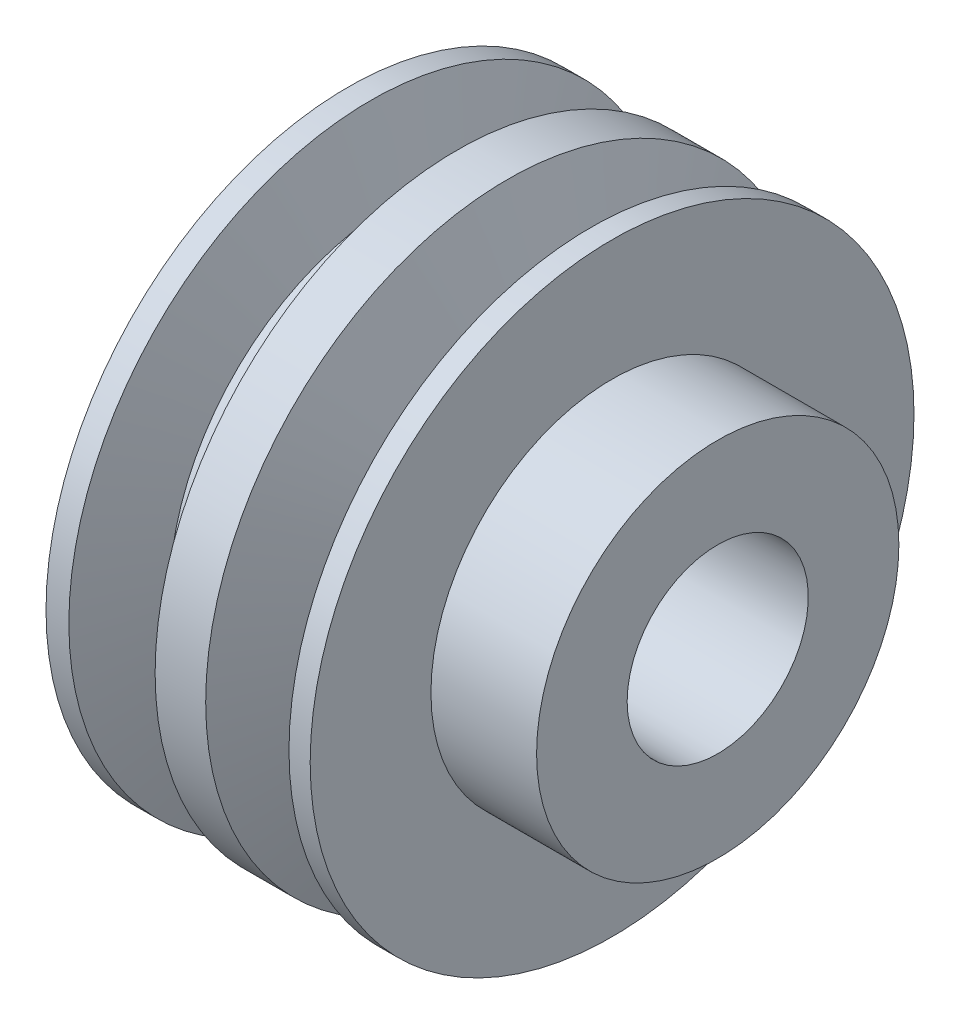
from build123d import *


with BuildPart() as part:
    # Sketch1 → Revolve1 (revolve)
    with BuildSketch(Plane(origin=(0, 0, 0), x_dir=(1, 0, 0), z_dir=(0, 1, 0)), mode=Mode.PRIVATE) as revolve1_sk:
        Polygon((0, 12), (0, 40), (3.025923231, 40), (6.441608618, 30.091710395), (11.827881728, 30.091710395), (14.455332026, 40), (21.155330284, 40), (25.227878246, 30.091710395), (28.774936147, 30.091710395), (32.190621534, 40), (35, 40), (35, 24), (48.996539792, 24), (48.996539792, 12), align=None)
    revolve(revolve1_sk.sketch.rotate(Axis((0, 0, 0), (1, 0, 0)), 180), axis=Axis((0, 0, 0), (1, 0, 0)))


solid = part.part
